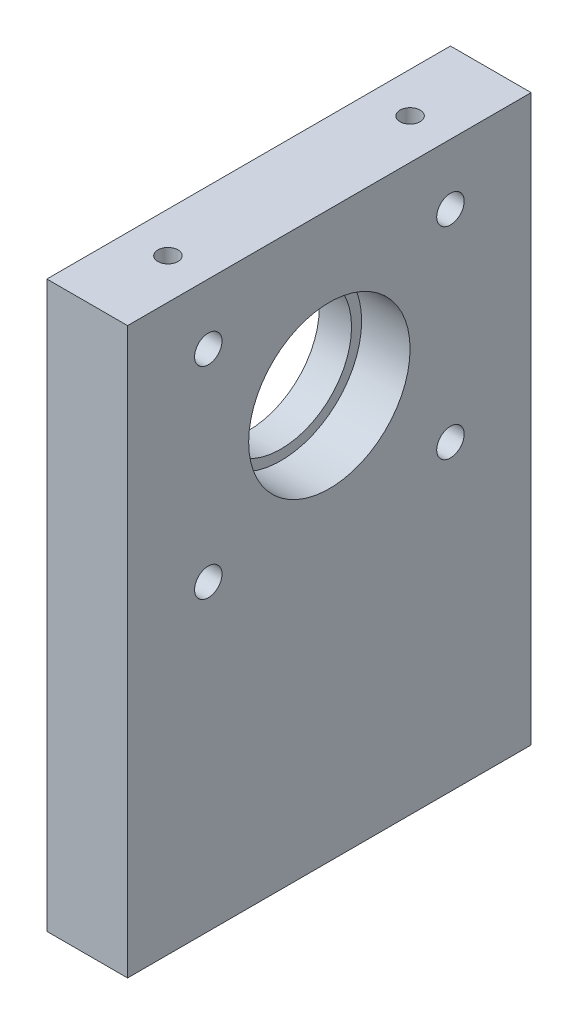
from build123d import *

# Parameters (mm, degrees)
SKETCH_1_W              = 100
SKETCH_1_H              = 140
EXTRUDE_1_DEPTH         = 20
HOLE_WIZARD_M10_1_D     = 8.5
HOLE_WIZARD_M10_1_DEPTH = 24.5
HOLE_WIZARD_M10_1_TIP   = 2.553657631
SKETCH_4_R              = 20
CUT_EXTRUDE_1_DEPTH     = 12
SKETCH_5_R              = 17.5
CUT_EXTRUDE_2_DEPTH     = 87.856203002
HOLE_WIZARD_M8_1_D      = 6.8
HOLE_WIZARD_M6_1_D      = 5
HOLE_WIZARD_M6_1_DEPTH  = 15
HOLE_WIZARD_M6_1_TIP    = 1.502151548


with BuildPart() as part:
    # 草图1 → 凸台-拉伸1 (new body)
    with BuildSketch(Plane(origin=(0, 0, 0), x_dir=(0, 0, -1), z_dir=(1, 0, 0))):
        Rectangle(SKETCH_1_W, SKETCH_1_H)
    extrude(amount=EXTRUDE_1_DEPTH)

    # M10 螺纹孔1
    with Locations(Plane(origin=(0, -70, 0), x_dir=(-1, 0, 0), z_dir=(0, -1, 0))):
        with Locations((-10, 30), (-10, -30)):
            Hole(HOLE_WIZARD_M10_1_D / 2, depth=HOLE_WIZARD_M10_1_DEPTH)
            with Locations((0, 0, -(HOLE_WIZARD_M10_1_DEPTH + HOLE_WIZARD_M10_1_TIP / 2))):  # 118° drill point
                Cone(0, HOLE_WIZARD_M10_1_D / 2, HOLE_WIZARD_M10_1_TIP, mode=Mode.SUBTRACT)

    # 草图4 → 切除-拉伸1 (cut)
    with BuildSketch(Plane(origin=(20, 0, 0), x_dir=(0, 0, -1), z_dir=(1, 0, 0))):
        with Locations((0, 30)):
            Circle(SKETCH_4_R)
    extrude(amount=-CUT_EXTRUDE_1_DEPTH, mode=Mode.SUBTRACT)

    # 草图5 → 切除-拉伸2 (cut, through all)
    with BuildSketch(Plane(origin=(8, 0, 0), x_dir=(0, 0, -1), z_dir=(1, 0, 0))):
        with Locations((0, 30)):
            Circle(SKETCH_5_R)
    extrude(amount=-CUT_EXTRUDE_2_DEPTH, mode=Mode.SUBTRACT)

    # M8 螺纹孔1 (through all)
    with Locations(Plane.ZY):
        with Locations((-30, 55), (30, 55), (-30, 5), (30, 5)):
            Hole(HOLE_WIZARD_M8_1_D / 2)

    # M6 螺纹孔1
    with Locations(Plane(origin=(0, 70, 0), x_dir=(1, 0, 0), z_dir=(0, 1, 0))):
        with Locations((10, 30), (10, -30)):
            Hole(HOLE_WIZARD_M6_1_D / 2, depth=HOLE_WIZARD_M6_1_DEPTH)
            with Locations((0, 0, -(HOLE_WIZARD_M6_1_DEPTH + HOLE_WIZARD_M6_1_TIP / 2))):  # 118° drill point
                Cone(0, HOLE_WIZARD_M6_1_D / 2, HOLE_WIZARD_M6_1_TIP, mode=Mode.SUBTRACT)


solid = part.part
